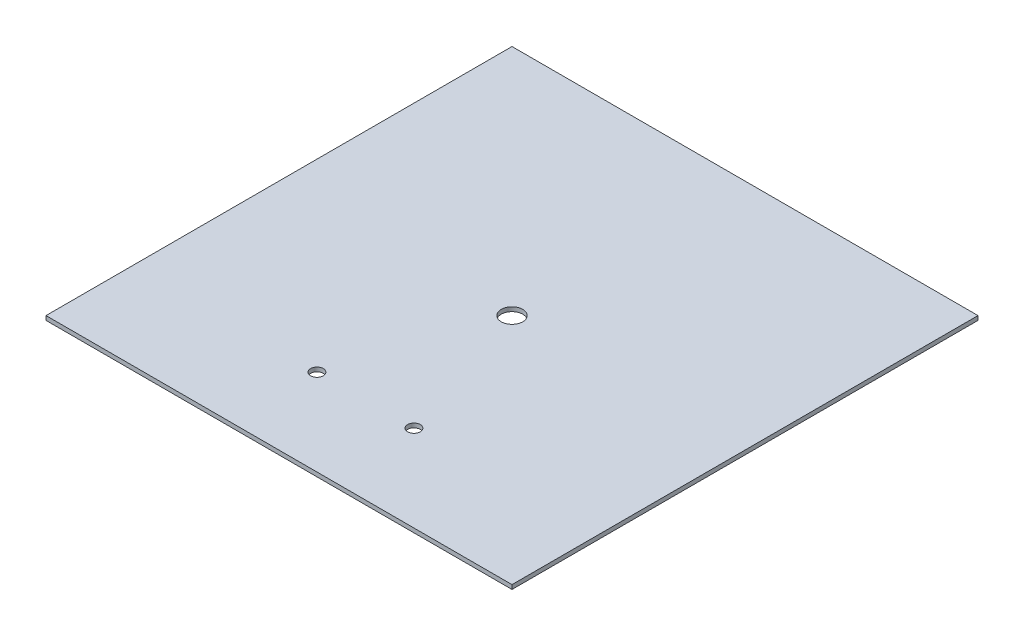
from build123d import *

# Parameters (mm, degrees)
SKETCH1_W           = 110.5
SKETCH1_H           = 110.5
SKETCH1_R           = 2.55
SKETCH1_R_2         = 1.5
BOSS_EXTRUDE1_DEPTH = 1


with BuildPart() as part:
    # Sketch1 → Boss-Extrude1 (new body)
    with BuildSketch(Plane(origin=(0, 0, 0), x_dir=(1, 0, 0), z_dir=(0, 1, 0))):
        Rectangle(SKETCH1_W, SKETCH1_H)
        with Locations(Location((0, 0, 0), (0, 0, 270))):
            Circle(SKETCH1_R, mode=Mode.SUBTRACT)
        with Locations(Location((-11.5, -34.75, 0), (0, 0, 270))):
            Circle(SKETCH1_R_2, mode=Mode.SUBTRACT)
        with Locations(Location((11.5, -34.75, 0), (0, 0, 270))):
            Circle(SKETCH1_R_2, mode=Mode.SUBTRACT)
    extrude(amount=BOSS_EXTRUDE1_DEPTH)


solid = part.part
